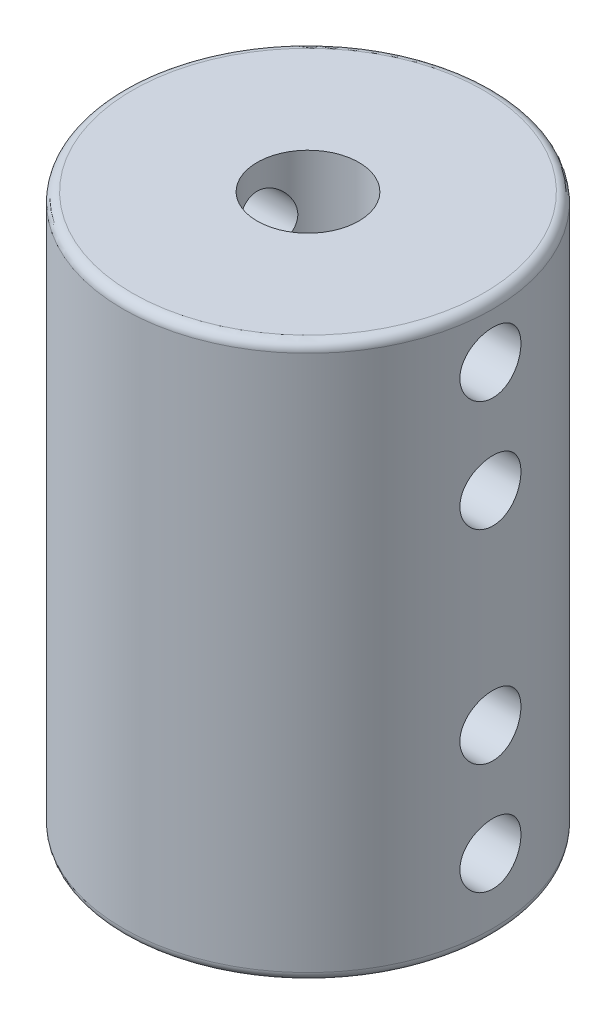
from build123d import *

# Parameters (mm, degrees)
SKETCH1_R           = 10
BOSS_EXTRUDE1_DEPTH = 30
SKETCH2_R           = 2.75
CUT_EXTRUDE1_DEPTH  = 15
SKETCH3_R           = 6
CUT_EXTRUDE2_DEPTH  = 15
M4_TAPPED_HOLE1_D   = 3.3
FILLET1_R           = 0.5


with BuildPart() as part:
    # Sketch1 → Boss-Extrude1 (new body)
    with BuildSketch(Plane(origin=(0, 0, 0), x_dir=(1, 0, 0), z_dir=(0, 1, 0))):
        with Locations(Location((0, 0, 0), (0, 0, 270))):
            Circle(SKETCH1_R)
    extrude(amount=BOSS_EXTRUDE1_DEPTH)

    # Sketch2 → Cut-Extrude1 (cut)
    with BuildSketch(Plane(origin=(0, 30, 0), x_dir=(1, 0, 0), z_dir=(0, 1, 0))):
        with Locations(Location((0, 0, 0), (0, 0, 270))):
            Circle(SKETCH2_R)
    extrude(amount=-CUT_EXTRUDE1_DEPTH, mode=Mode.SUBTRACT)

    # Sketch3 → Cut-Extrude2 (cut)
    with BuildSketch(Plane.XZ):
        with Locations(Location((0, 0, 0), (0, 0, 270))):
            Circle(SKETCH3_R)
    extrude(amount=-CUT_EXTRUDE2_DEPTH, mode=Mode.SUBTRACT)

    # M4 Tapped Hole1 (through all)
    with Locations(Plane(origin=(10, 4, 0), x_dir=(0, 0, 1), z_dir=(1, 0, 0))):
        with Locations((0, 0), (0, -6), (0, -23), (0, -17)):
            Hole(M4_TAPPED_HOLE1_D / 2)

    # Fillet1
    fillet1_edges = [part.edges().sort_by_distance(p)[0] for p in [
        (0, 0, -10),
        (0, 30, -10),
    ]]
    fillet(fillet1_edges, radius=FILLET1_R)


solid = part.part
